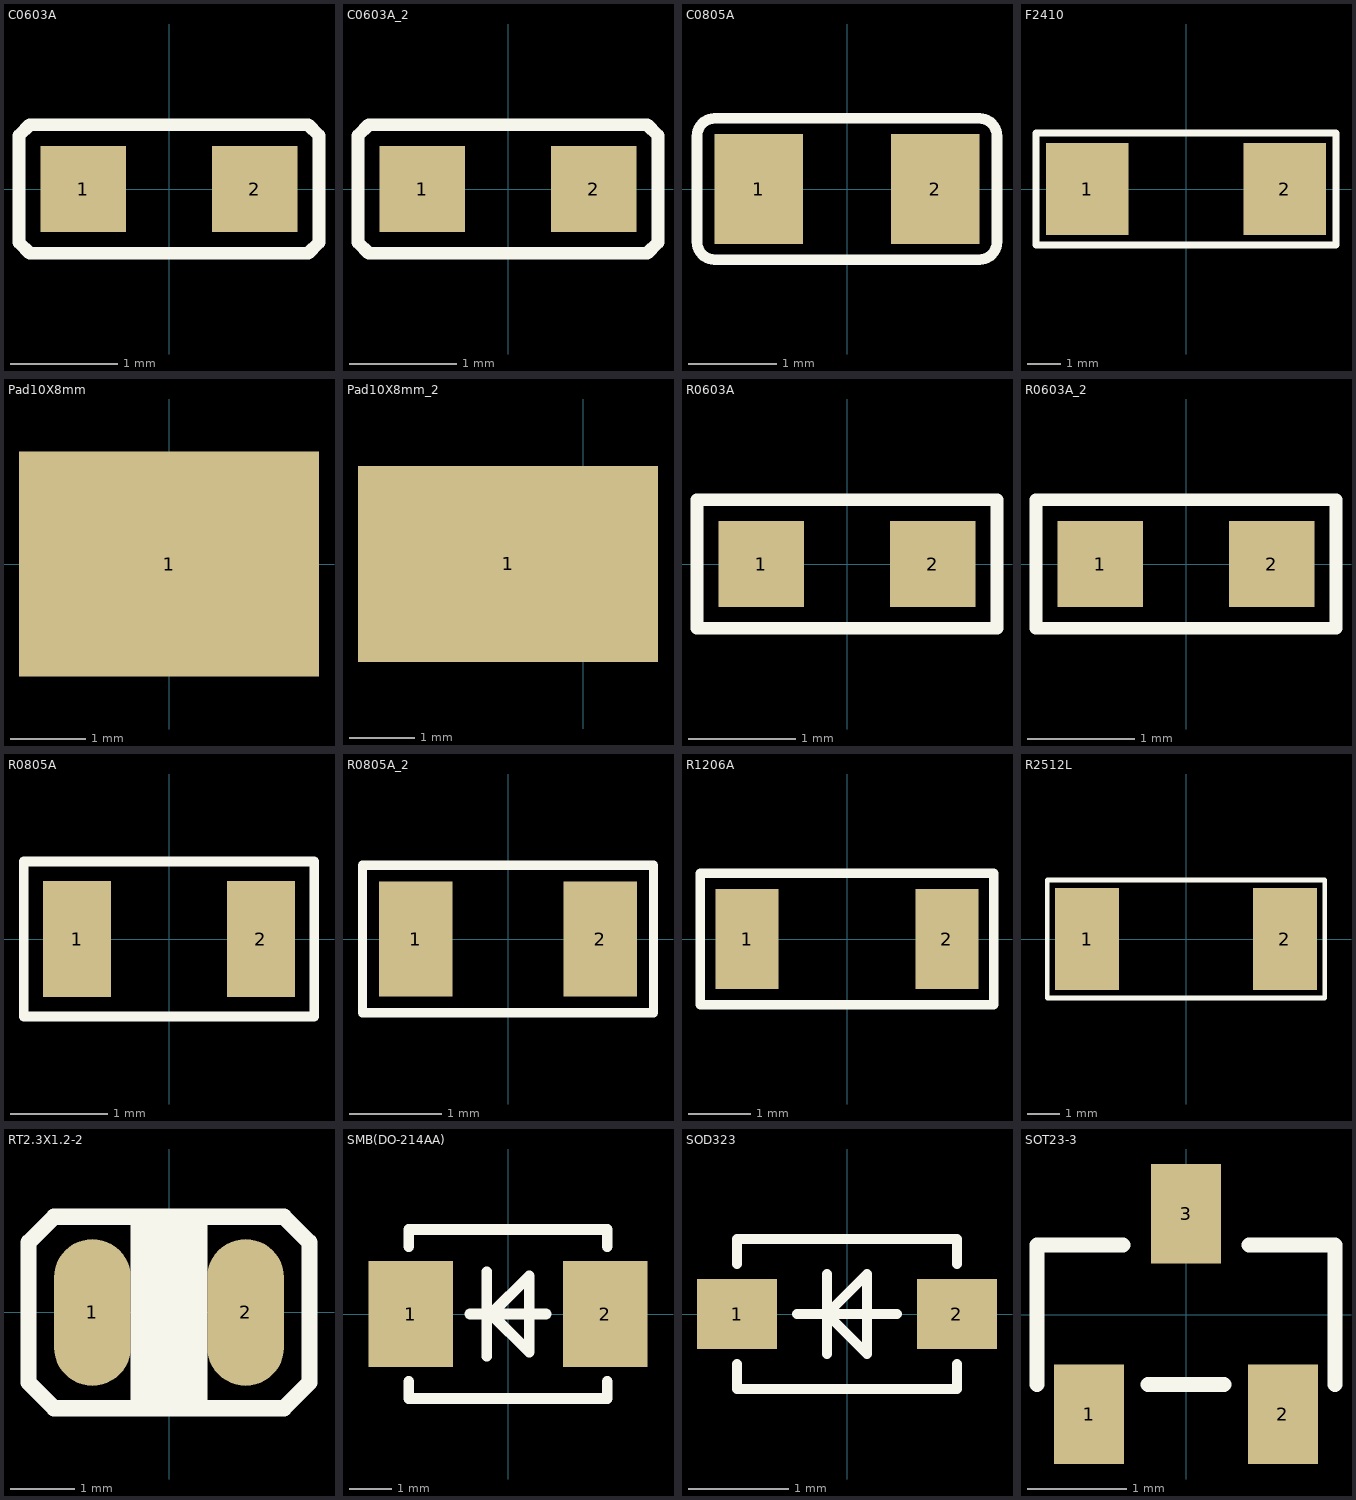
[diagram p0: the footprints below, top view; thin cyan lines are the x and y axes]
# Altium footprint library MISC84401-2.PcbLib: 19 footprints (part 1 of 2)
Each footprint in its own frame and in the unit in brackets; x right, y up, seen from the top. Pads: shape width x height; smd on the part's side, far side on the other; paste and mask are expansions set on the pad; w line width, h text height; cw(c..) or ccw(c..) is an arc to the next point about the centre after c.

## C0603A [mm] "SMD capacitor"
pads (2):
  rect 0.8x0.8 smd mask+0.08: 1(-0.8,0) 2(0.8,0)
Top Overlay:
  lines w0.12: 0.551,-0.6 1.2,-0.6 ; -1.4,-0.5 -1.3,-0.6 1.3,-0.6 1.4,-0.5 1.4,0.5 1.3,0.6 -1.3,0.6 -1.4,0.5 -1.4,-0.5

## C0603A_2 [mm]
pads (2):
  rect 0.8x0.8 smd mask+0.08: 1(-0.8,0) 2(0.8,0)
Top Overlay:
  lines w0.12: 0.551,-0.6 1.2,-0.6 ; -1.4,-0.5 -1.3,-0.6 1.3,-0.6 1.4,-0.5 1.4,0.5 1.3,0.6 -1.3,0.6 -1.4,0.5 -1.4,-0.5

## C0805A [mm] "SMD capacitor"
height 10
pads (2):
  rect 1x1.25 smd: 1(-1,0)
  rect 1x1.25 smd mask+0.102: 2(1,0)
Top Overlay:
  lines w0.12: -1.7,-0.6 ccw(c-1.5,-0.6) -1.5,-0.8 1.5,-0.8 ccw(c1.5,-0.6) 1.7,-0.6 1.7,0.6 ccw(c1.5,0.6) 1.5,0.8 -1.5,0.8 ccw(c-1.5,0.6) -1.7,0.6 -1.7,-0.6

## F2410 [mm] "SMD fuse"
height 10
pads (2):
  rect 2.5x2.8 smd: 1(-3,0) 2(3,0)
Top Overlay:
  lines w0.2: -4.55,-1.7 4.55,-1.7 4.55,1.7 -4.55,1.7 -4.55,-1.7

## Pad10X8mm [mm]
pads (1):
  rect 4x3 smd: 1(0,0)

## Pad10X8mm_2 [mm]
pads (1):
  rect 4.6x3 smd: 1(-1.154,-7.524)

## R0603A [mm] "SMD resistor"
height 0.5
pads (2):
  rect 0.8x0.8 smd mask+0.08: 1(-0.8,0) 2(0.8,0)
Top Overlay:
  lines w0.12: -1.4,-0.6 1.4,-0.6 1.4,0.6 -1.4,0.6 -1.4,-0.6

## R0603A_2 [mm]
pads (2):
  rect 0.8x0.8 smd mask+0.08: 1(-0.8,0) 2(0.8,0)
Top Overlay:
  lines w0.12: -1.4,-0.6 1.4,-0.6 1.4,0.6 -1.4,0.6 -1.4,-0.6

## R0805A [mm] "SMD resistor"
pads (2):
  rect 0.7x1.2 smd paste+0 mask+0.08: 1(-0.95,0) 2(0.95,0)
Top Overlay:
  lines w0.1: -1.5,-0.8 -1.5,0.8 1.5,0.8 1.5,-0.8 -1.5,-0.8

## R0805A_2 [mm]
pads (2):
  rect 0.8x1.25 smd paste+0 mask+0.08: 1(-1,0) 2(1,0)
Top Overlay:
  lines w0.1: -1.575,-0.8 -1.575,0.8 1.575,0.8 1.575,-0.8 -1.575,-0.8

## R1206A [mm] "SMD resistor"
pads (2):
  rect 1x1.6 smd: 1(-1.6,0) 2(1.6,0)
Top Overlay:
  lines w0.15: -2.35,-1.05 -2.35,1.05 2.35,1.05 2.35,-1.05 -2.35,-1.05

## R2512L [mm] "SMD resistor"
height 10
pads (2):
  rect 2x3.2 smd: 1(-3.1,0) 2(3.1,0)
Top Overlay:
  lines w0.15: -4.35,-1.85 4.35,-1.85 4.35,1.85 -4.35,1.85 -4.35,-1.85

## RT2.3X1.2-2 [mm] "Wire-soldered NTC"
pads (2):
  oval 1.2x2.3 smd: 1(-1.2,0) 2(1.2,0)
Top Overlay:
  rectangle: -0.6,-1.55 0.6,1.5
  lines w0.254: -2.2,-1.075 -2.2,1.075 ; -2.2,1.1 -1.8,1.5 ; 2.2,-1.075 2.2,1.075 ; 2.2,1.1 1.8,1.5 -1.8,1.5 ; -2.2,-1.1 -2.2,-1.1 ; -2.2,-1.1 -1.8,-1.5 ; -1.8,-1.5 1.8,-1.5 2.2,-1.1 ; -1.8,-1.5 -1.8,-1.5 ; -1.8,1.5 -1.8,1.5 ; 2.2,-1.1 2.2,-1.1

## SMB(DO-214AA) [mm] "SMD diode"
height 10
pads (2):
  rect 2x2.5 smd: 1(-2.3,0) 2(2.3,0)
Top Overlay:
  lines w0.254: -2.35,-1.6 -2.35,-2 2.35,-2 2.35,-1.6 ; -2.35,1.6 -2.35,2 2.35,2 2.35,1.6 ; -0.9,0 0.9,0 ; -0.5,-1 -0.5,1 ; -0.4,0 0.5,-0.9 0.5,0.9 -0.4,0

## SOD323 [mm] "SMD diode"
pads (2):
  rect 0.8x0.7 smd: 1(-1.1,0) 2(1.1,0)
Top Overlay:
  lines w0.1: -1.1,-0.5 -1.1,-0.75 1.1,-0.75 1.1,-0.5 ; -1.1,0.5 -1.1,0.75 1.1,0.75 1.1,0.5 ; -0.5,0 0.5,0 ; -0.2,-0.4 -0.2,0.4 ; -0.2,0 0.2,-0.4 0.2,0.4 -0.2,0

## SOT23-3 [mm] "SMD IC/MOS*"
pads (3):
  rect 0.7x1 smd: 1(-0.975,-1) 2(0.975,-1) 3(0,1.016)
Top Overlay:
  lines w0.15: -1.5,-0.7 -1.5,0.7 -0.635,0.7 ; -0.381,-0.7 0.381,-0.7 ; 0.635,0.7 1.5,0.7 1.5,-0.7